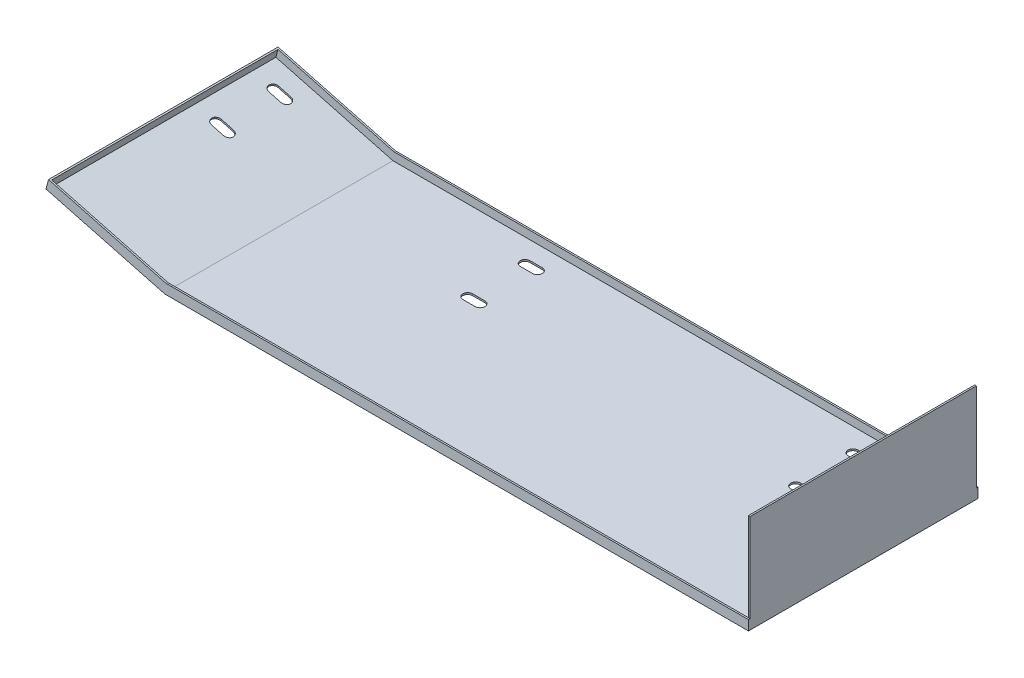
SolidWorks part; units mm, degrees
material "Plain Carbon Steel"
ref_plane "Front Plane" through (0, 0, 0) normal (0, 0, 1) x (1, 0, 0)
ref_plane "Top Plane" through (0, 0, 0) normal (0, 1, 0) x (1, 0, 0)
ref_plane "Right Plane" through (0, 0, 0) normal (1, 0, 0) x (0, 0, -1)
sketch "Sketch1" plane through (0, 0, 0) normal (0, 0, 1) x (1, 0, 0)
  line L0 (0, 0) -> (0, 120)
  line L1 (0, 0) -> (-712, 0)
  line L2 (-712, 0) -> (-856.99, 38.4434)
  dimension "D1" = 120
  dimension "D2" = 712
  dimension "D3" = 150
  dimension "D4" = 165.15
extrude "Extrude-Thin1" add sketch "Sketch1" along normal blind 276 thin thin type one direction wall 2
sketch "Sketch2" plane through (0, 0, 276) normal (0, 0, 1) x (1, 0, 0)
  line L1 (-712, 0) -> (-856.99, 38.4434)
  line L3 (0, 0) -> (-712, 0)
extrude "Extrude-Thin2" add sketch "Sketch2" along normal blind 2 thin
sketch "Sketch4" plane through (0, 0, 0) normal (0, 0, -1) x (-1, 0, 0)
  line L0 (0, 0) -> (712, 0)
  line L1 (712, 0) -> (856.99, 38.4434)
extrude "Extrude-Thin3" add sketch "Sketch4" along normal blind 2 thin thin type one direction reverse wall 12
sketch "Sketch5" plane through (0, 0, 0) normal (0, -1, 0) x (1, 0, 0)
  line L0 (-122.5, 28) -> (-107.5, 28) construction
  line L1 (-122.5, 34) -> (-107.5, 34)
  line L2 (-122.5, 22) -> (-107.5, 22)
  line L4 (0, 278) -> (0, -2) construction
  line L5 (0, -2) -> (-712, -2) construction
  arc A0 (-122.5, 34) -> (-122.5, 22) centre (-122.5, 28) ccw
  arc A1 (-107.5, 22) -> (-107.5, 34) centre (-107.5, 28) ccw
  point P2 (-115, 28)
  dimension "D1" = 6
  dimension "D2" = 15
  dimension "D3" = 30
  dimension "D4" = 115
extrude "Cut-Extrude1" cut sketch "Sketch5" against normal blind 2
sketch "Sketch6" plane through (-46.7672, -176.3833, 0) normal (-0.2563, -0.9666, 0) x (0.9666, -0.2563, 0)
  line L0 (-809.7193, 28) -> (-794.7193, 28) construction
  line L1 (-809.7193, 34) -> (-794.7193, 34)
  line L2 (-809.7193, 22) -> (-794.7193, 22)
  line L4 (-688.2193, 278) -> (-688.2193, -2) construction
  line L5 (-688.2193, -2) -> (-838.2193, -2) construction
  arc A0 (-809.7193, 34) -> (-809.7193, 22) centre (-809.7193, 28) ccw
  arc A1 (-794.7193, 22) -> (-794.7193, 34) centre (-794.7193, 28) ccw
  point P2 (-802.2193, 28)
  dimension "D1" = 6
  dimension "D2" = 15
  dimension "D3" = 30
  dimension "D4" = 114
extrude "Cut-Extrude2" cut sketch "Sketch6" against normal blind 2
sketch "Sketch7" plane through (-46.2546, -174.4501, 0) normal (0.2563, 0.9666, 0) x (0.9666, -0.2563, 0)
  line L0 (-688.4799, -276) -> (-838.2193, -276) construction
  line L1 (-838.2193, 0) -> (-836.2193, 0)
  line L2 (-838.2193, 0) -> (-838.2193, -276)
  line L3 (-838.2193, -276) -> (-836.2193, -276)
  line L4 (-836.2193, 0) -> (-836.2193, -276)
  dimension "D1" = 2
extrude "Boss-Extrude1" add sketch "Sketch7" along normal blind 10
pattern_linear "LPattern1" count 2 spacing 70 along (0, 0, 1) of "Cut-Extrude2"
pattern_linear "LPattern2" count 2 spacing 70 along (0, 0, 1) count 2 spacing 400 along (-1, 0, 0) of "Cut-Extrude1"
